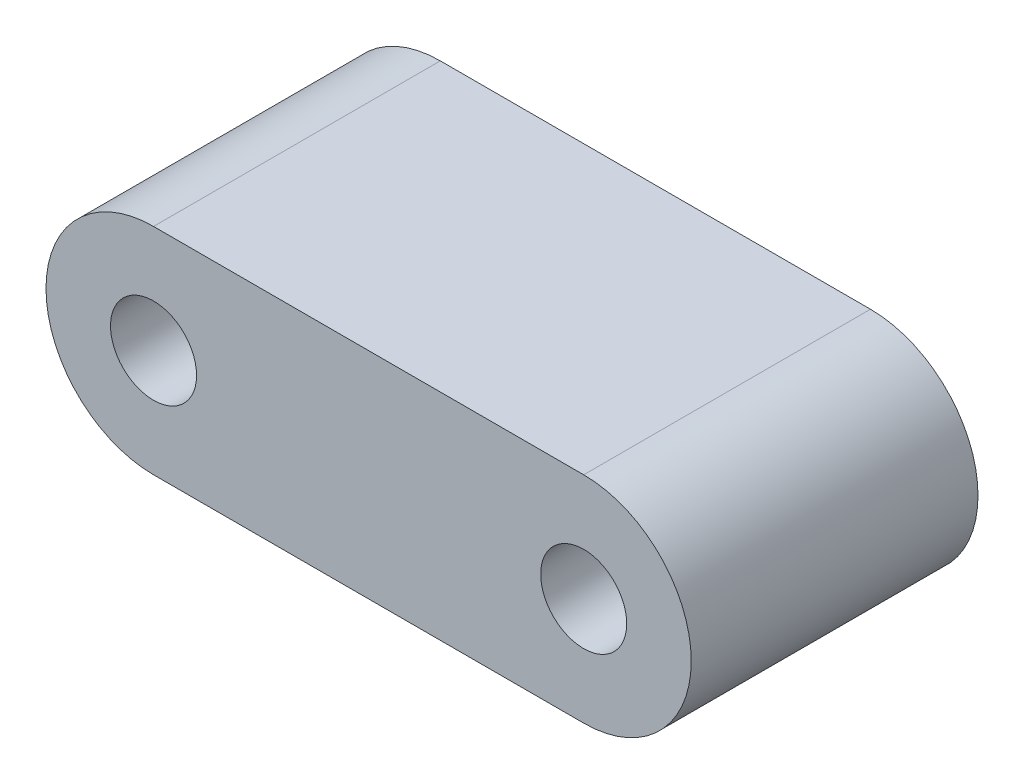
from build123d import *

# Parameters (mm, degrees)
SKETCH1_R           = 3
BOSS_EXTRUDE1_DEPTH = 20


with BuildPart() as part:
    # Sketch1 → Boss-Extrude1 (new body)
    with BuildSketch(Plane.XY):
        with BuildLine():
            Line((0, 7.5), (30, 7.5))
            ThreePointArc((30, 7.5), (37.5, 0), (30, -7.5))
            Line((30, -7.5), (0, -7.5))
            ThreePointArc((0, -7.5), (-7.5, 0), (0, 7.5))
        make_face()
        Circle(SKETCH1_R, mode=Mode.SUBTRACT)
        with Locations((30, 0)):
            Circle(SKETCH1_R, mode=Mode.SUBTRACT)
    extrude(amount=BOSS_EXTRUDE1_DEPTH)


solid = part.part
